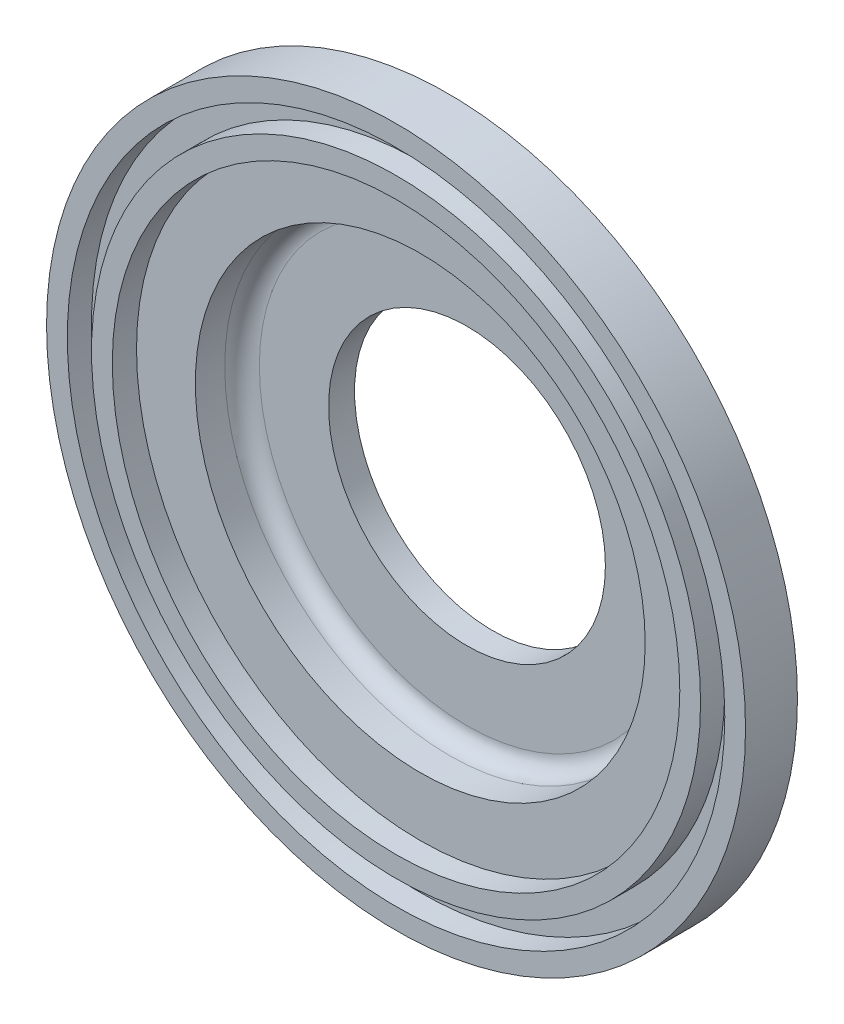
SolidWorks part; units mm, degrees
material "灰铸铁 HT150 "
ref_plane "Front Plane" through (0, 0, 0) normal (0, 0, 1) x (1, 0, 0)
ref_plane "Top Plane" through (0, 0, 0) normal (0, 1, 0) x (1, 0, 0)
ref_plane "Right Plane" through (0, 0, 0) normal (1, 0, 0) x (0, 0, -1)
sketch "Sketch1" plane through (0, 0, 0) normal (1, 0, 0) x (0, 0, -1)
  line L0 (0, 0) -> (110.7692, 0) construction
  line L1 (0, 164) -> (0, 176)
  line L2 (0, 202) -> (30, 202)
  line L3 (30, 202) -> (30, 145)
  line L4 (30, 145) -> (56, 145)
  line L5 (56, 145) -> (56, 80)
  line L6 (56, 80) -> (41, 80)
  line L7 (41, 80) -> (41, 130)
  line L8 (41, 130) -> (14, 130)
  line L9 (14, 130) -> (14, 164)
  line L10 (14, 164) -> (0, 164)
  line L15 (0, 190) -> (0, 202)
  line L16 (0, 190) -> (14, 190)
  line L17 (0, 176) -> (14, 176)
  line L18 (14, 190) -> (14, 176)
  dimension "D1" = 80
  dimension "D2" = 130
  dimension "D3" = 164
  dimension "D4" = 176
  dimension "D5" = 190
  dimension "D6" = 202
  dimension "D7" = 14
  dimension "D8" = 56
  dimension "D9" = 15
  dimension "D10" = 30
  dimension "D11" = 145
revolve "Revolve1" add sketch "Sketch1" angle 360 about L0
fillet "Fillet1" radius 10 1 edges at (130, 0, -41)
